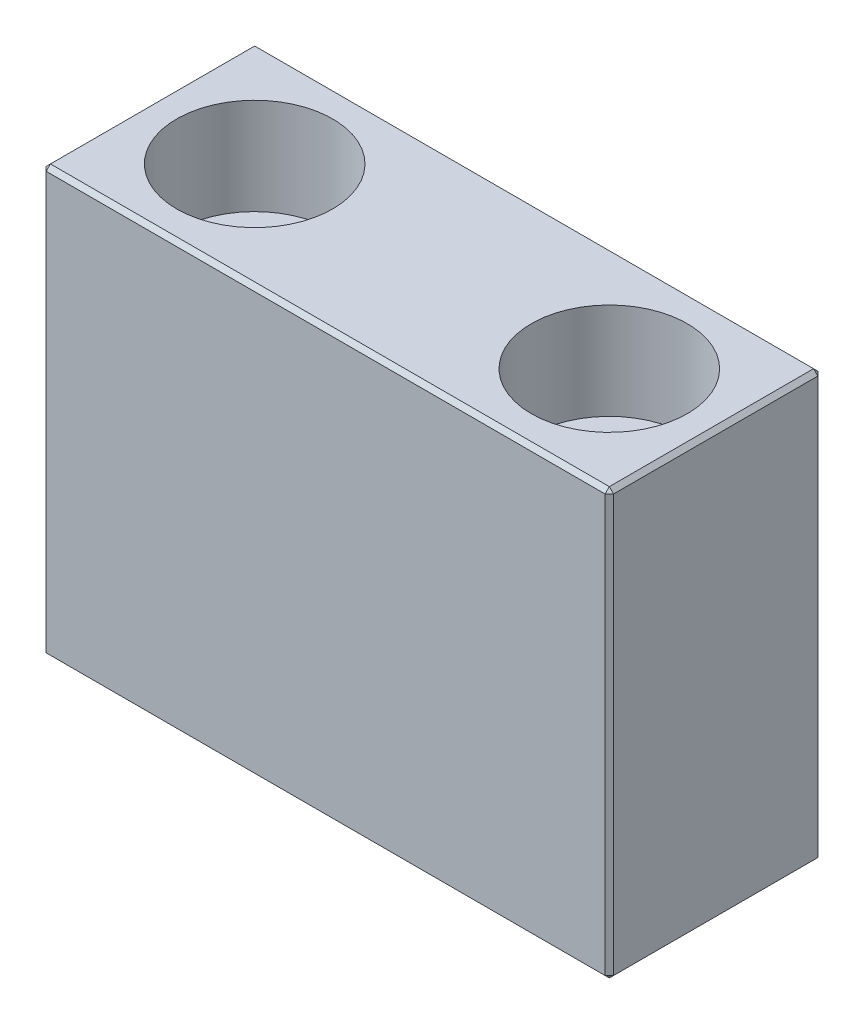
from build123d import *

# Parameters (mm, degrees)
SKETCH_1_W                = 40
SKETCH_1_H                = 30
EXTRUDE_1_DEPTH           = 15
HOLE_WIZARD_1_D           = 6.6
HOLE_WIZARD_1_CBORE_D     = 11
HOLE_WIZARD_1_CBORE_DEPTH = 6.8
CHAMFER_1_SIZE            = 0.3


with BuildPart() as part:
    # 草图1 → 凸台-拉伸1 (new body)
    with BuildSketch(Plane.XY):
        Rectangle(SKETCH_1_W, SKETCH_1_H)
    extrude(amount=EXTRUDE_1_DEPTH)

    # 打孔尺寸根据内六角圆柱头螺钉的类型1 (through all)
    with Locations(Plane(origin=(0, 15, 0), x_dir=(1, 0, 0), z_dir=(0, 1, 0))):
        with Locations((-12.5, -7.5), (12.5, -7.5)):
            CounterBoreHole(HOLE_WIZARD_1_D / 2, HOLE_WIZARD_1_CBORE_D / 2, HOLE_WIZARD_1_CBORE_DEPTH)

    # 倒角1
    chamfer_1_edges = [part.edges().sort_by_distance(p)[0] for p in [
        (-20, 0, 15),
        (0, -15, 15),
        (20, 0, 15),
        (0, -15, 0),
        (-20, 0, 0),
        (0, 15, 0),
        (20, 0, 0),
        (0, 15, 15),
        (20, -15, 7.5),
        (-20, -15, 7.5),
        (-20, 15, 7.5),
        (20, 15, 7.5),
    ]]
    chamfer(chamfer_1_edges, length=CHAMFER_1_SIZE)


solid = part.part
